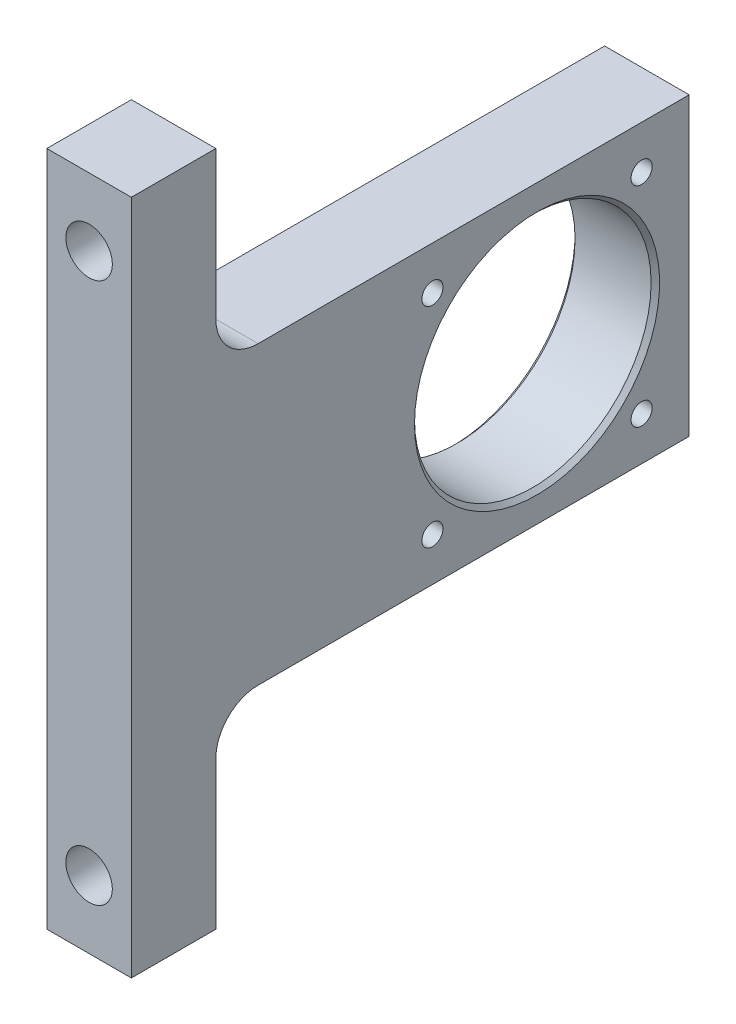
from build123d import *

# Parameters (mm, degrees)
BOSS_EXTRUDE1_DEPTH        = 10
SKETCH2_R                  = 14
CUT_EXTRUDE1_DEPTH         = 78.820305833
F_5_5_5_5_DIAMETER_HOLE1_D = 5.5
M3_TAPPED_HOLE1_D          = 2.5
FILLET1_R                  = 5
CHAMFER1_SIZE              = 0.5


with BuildPart() as part:
    # Sketch1 → Boss-Extrude1 (new body)
    with BuildSketch(Plane(origin=(0, 0, 0), x_dir=(0, 0, -1), z_dir=(1, 0, 0))):
        Polygon((0, -40), (0, 40), (10, 40), (10, 17.5), (66, 17.5), (66, -17.5), (10, -17.5), (10, -40), align=None)
    extrude(amount=BOSS_EXTRUDE1_DEPTH)

    # Sketch2 → Cut-Extrude1 (cut, through all)
    with BuildSketch(Plane(origin=(10, 0, 0), x_dir=(0, 0, -1), z_dir=(1, 0, 0))):
        with Locations((48, 0)):
            Circle(SKETCH2_R)
    extrude(amount=-CUT_EXTRUDE1_DEPTH, mode=Mode.SUBTRACT)

    # Ø5.5 (5.5) Diameter Hole1 (through all)
    with Locations(Plane.XY):
        with Locations((5, 32), (5, -32)):
            Hole(F_5_5_5_5_DIAMETER_HOLE1_D / 2)

    # M3 Tapped Hole1 (through all)
    with Locations(Plane(origin=(10, 0, 0), x_dir=(0, 0, -1), z_dir=(1, 0, 0))):
        with Locations((35.625631329, 12.374368671), (60.374368671, 12.374368671), (60.374368671, -12.374368671), (35.625631329, -12.374368671)):
            Hole(M3_TAPPED_HOLE1_D / 2)

    # Fillet1
    fillet1_edges = [part.edges().sort_by_distance(p)[0] for p in [
        (5, 17.5, -10),
        (5, -17.5, -10),
    ]]
    fillet(fillet1_edges, radius=FILLET1_R)

    # Chamfer1
    chamfer1_edges = [part.edges().sort_by_distance(p)[0] for p in [
        (0, 0, -34),
        (10, 0, -34),
    ]]
    chamfer(chamfer1_edges, length=CHAMFER1_SIZE)


solid = part.part
